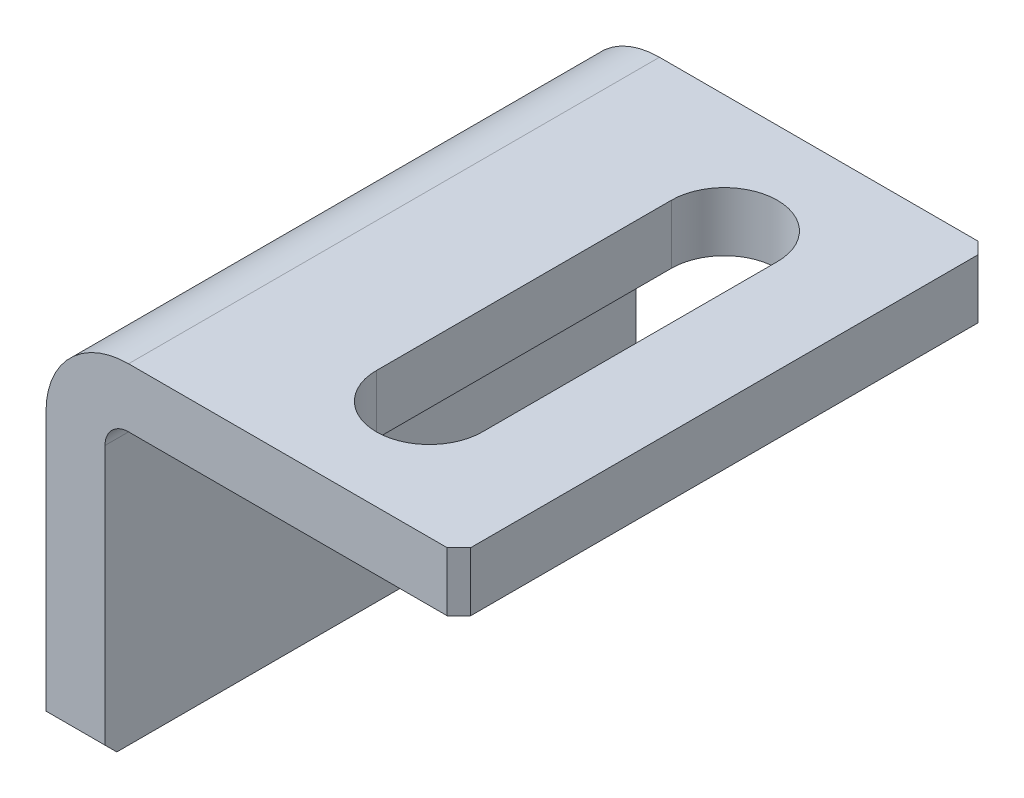
from build123d import *

# Parameters (mm, degrees)
EXTRUDE_1_DEPTH     = 45
CUT_EXTRUDE_1_DEPTH = 63.24949799
FILLET_1_R          = 2
FILLET_2_R          = 7
CHAMFER_1_SIZE      = 1


with BuildPart() as part:
    # 草图1 → 拉伸-薄壁1 (new body)
    with BuildSketch(Plane.XY):
        Polygon((0, 0), (0, 30), (35, 30), (35, 25), (5, 25), (5, 0), align=None)
    extrude(amount=EXTRUDE_1_DEPTH)

    # 草图2 → 切除-拉伸1 (cut, through all)
    with BuildSketch(Plane.XZ.offset(-25)):
        with BuildLine():
            Line((27, 35), (27, 10))
            ThreePointArc((27, 10), (22.5, 5.5), (18, 10))
            Line((18, 10), (18, 35))
            ThreePointArc((18, 35), (22.5, 39.5), (27, 35))
        make_face()
    extrude(amount=-CUT_EXTRUDE_1_DEPTH, mode=Mode.SUBTRACT)

    # 圆角1
    fillet_1_edges = [part.edges().sort_by_distance(p)[0] for p in [
        (5, 25, 22.5),
    ]]
    fillet(fillet_1_edges, radius=FILLET_1_R)

    # 圆角2
    fillet_2_edges = [part.edges().sort_by_distance(p)[0] for p in [
        (0, 30, 22.5),
    ]]
    fillet(fillet_2_edges, radius=FILLET_2_R)

    # 倒角1
    chamfer_1_edges = [part.edges().sort_by_distance(p)[0] for p in [
        (2.5, 0, 45),
        (2.5, 0, 0),
        (35, 27.5, 0),
        (35, 27.5, 45),
    ]]
    chamfer(chamfer_1_edges, length=CHAMFER_1_SIZE)


solid = part.part
